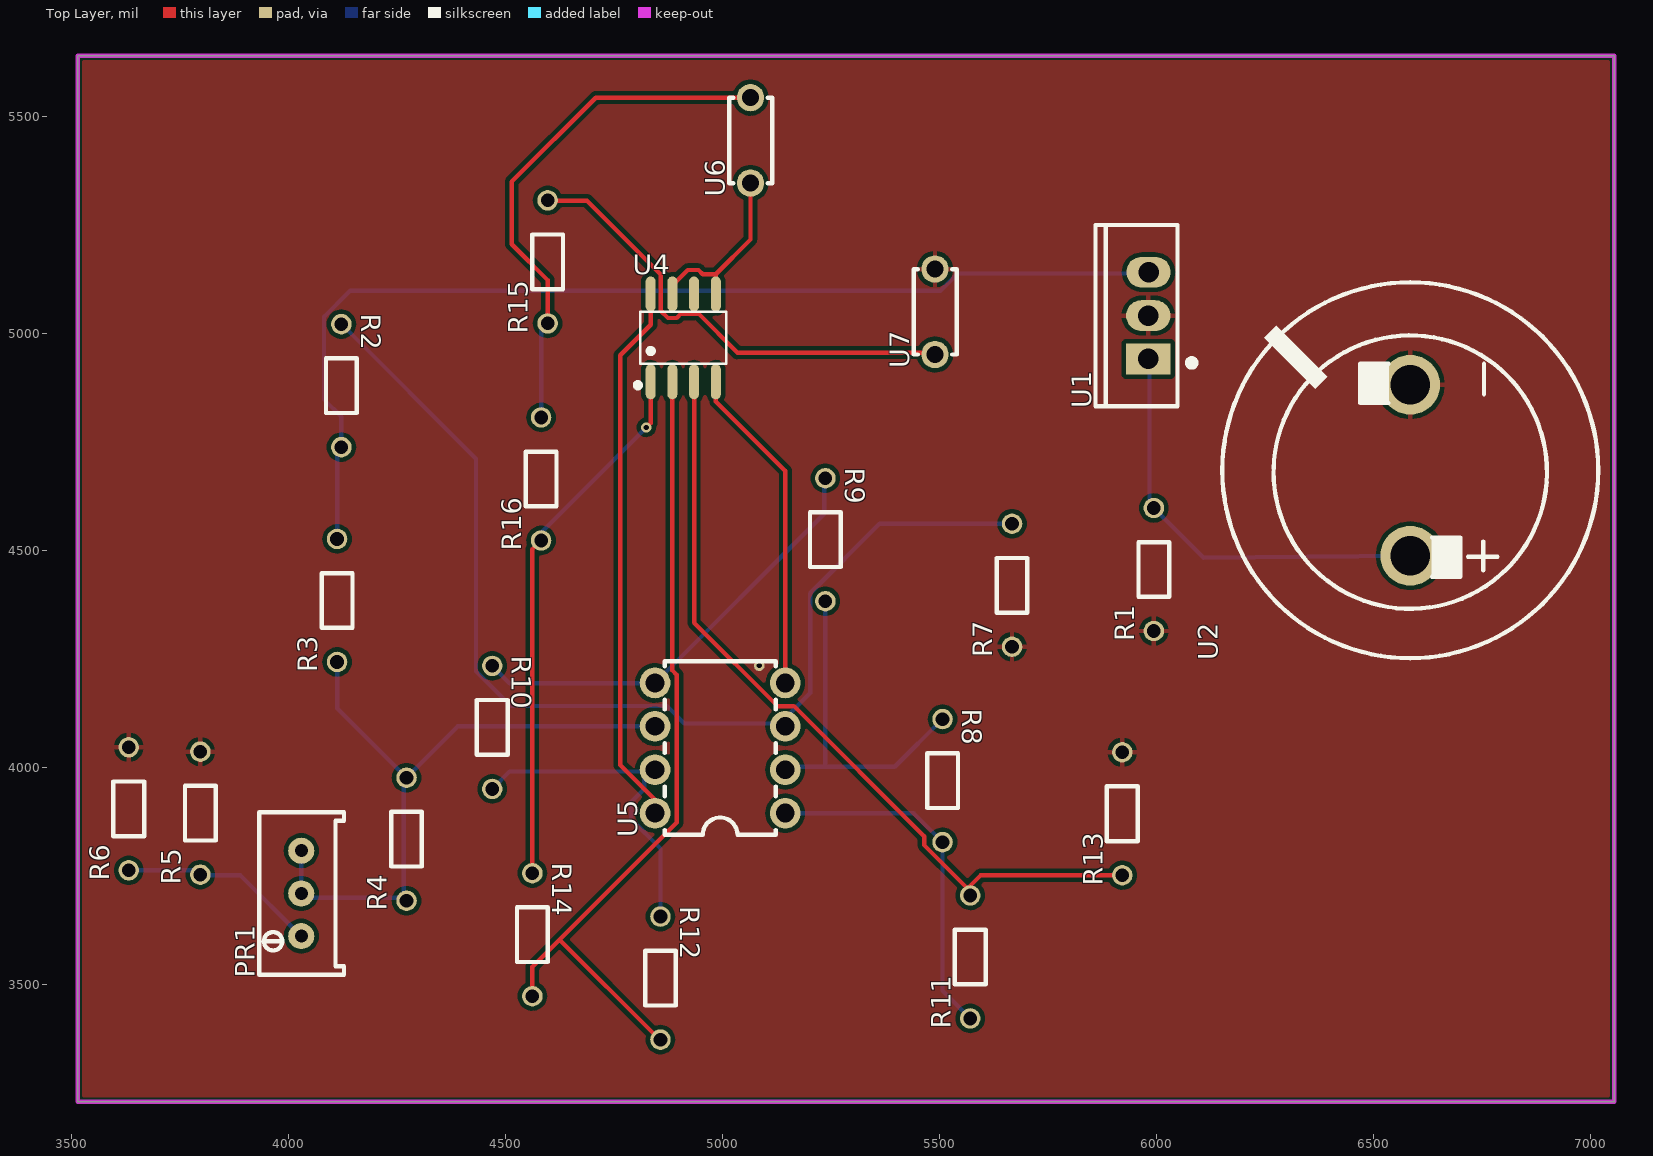
[diagram p0: Top Layer view]
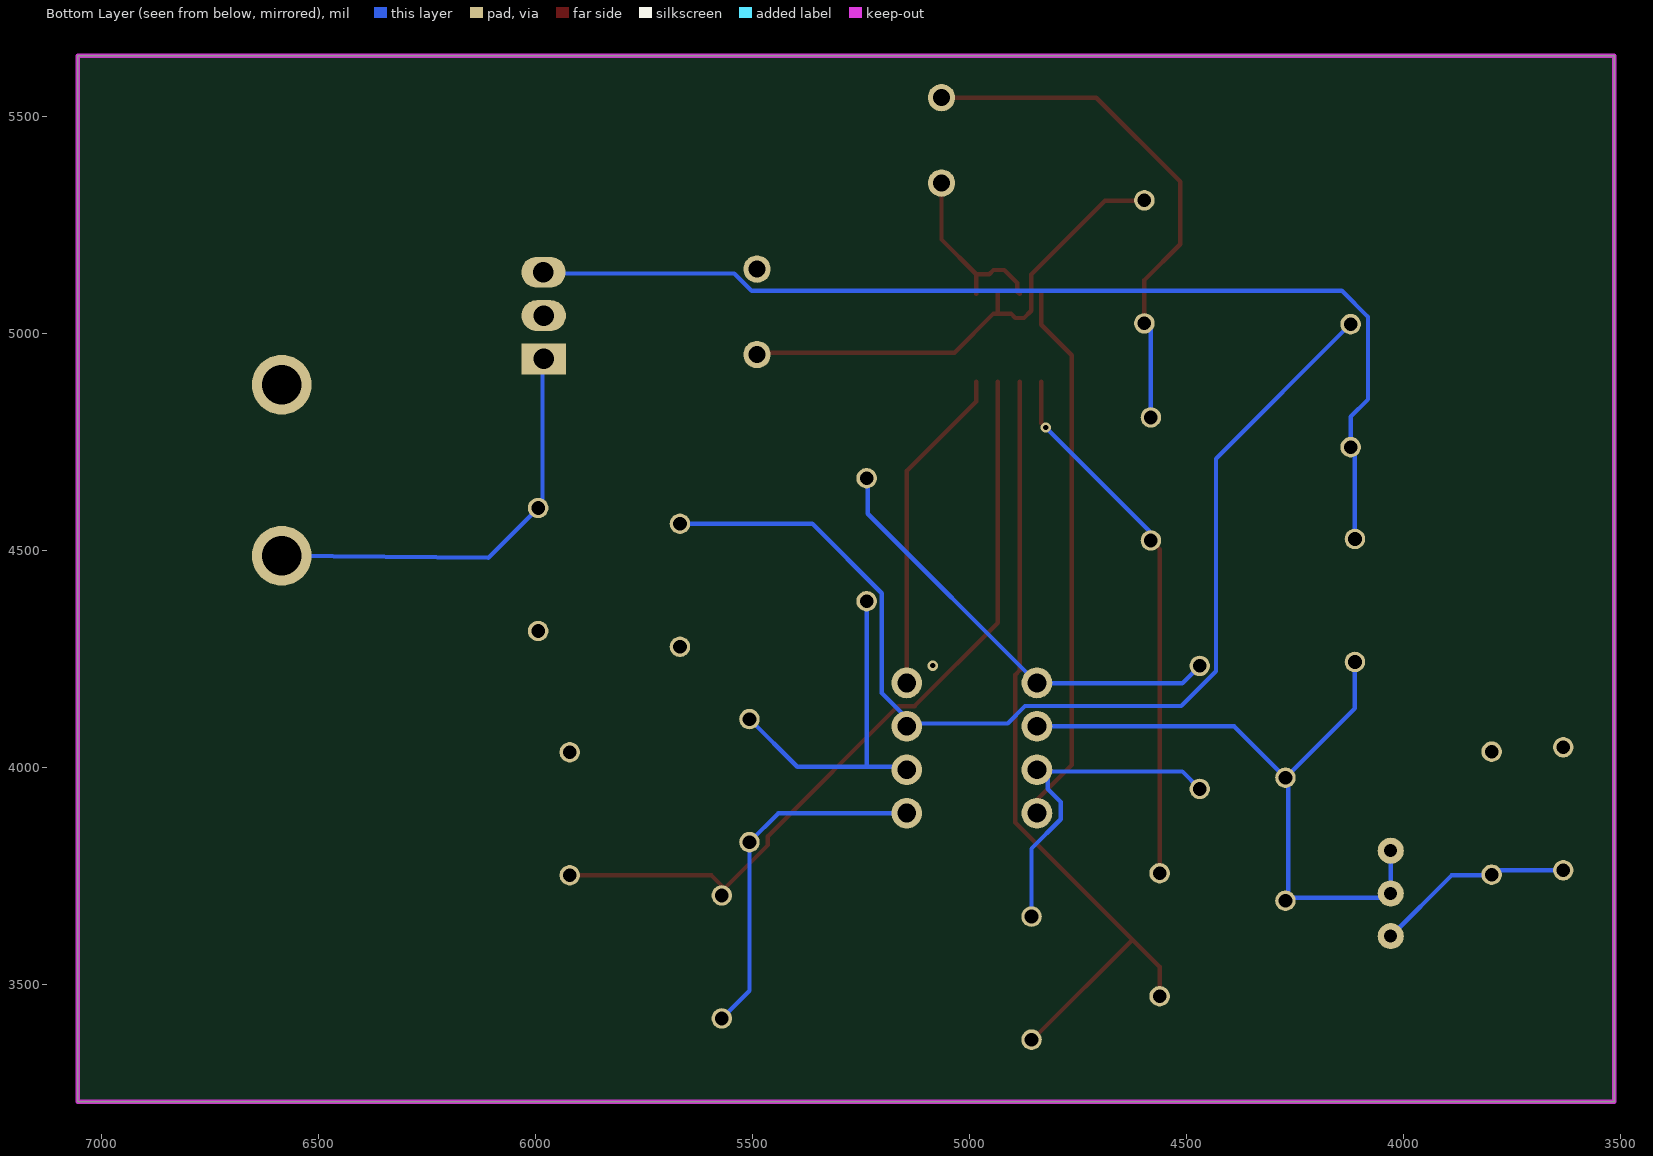
[diagram p1: Bottom Layer view, seen from below]
# Altium PCB MISC51804.pcbdoc
Units mil, origin at the board's own origin, x right, y up, seen from the top; angles counter-clockwise.
Board outline 3540 x 2410 mil, 2 copper layers (Top Layer, Bottom Layer), stack 62.206 mil thick; 23 components, 18 nets, 60 pads, 2 vias.

## Layer stack, top to bottom
Top Solder Mask Layer: solder mask 0.394, Dk 3.3
Top Layer: signal copper 1.379
Dielectric1: surface 59.449, FR4, Dk 4.5
Bottom Layer: signal copper 1.378
Bottom Solder Mask Layer: solder mask 0.394, Dk 3.3

## Board outline
3515,5640 3515,3230 7055,3230 7055,5640

## Design rules (kind name [scope] priority, off if disabled: settings)
BoardOutlineClearance copperThickness2oz_1 [All] p2 off: genericclearance=7.99 ignorepadtopadclearanceinfootprint=FALSE except(0: Arc-SplitContinuation Track-SplitContinuation SMDPad-SplitContinuation THPad-SplitContinuation Via-SplitContinuation Fill-SplitContinuation Region-SplitContinuation Poly-SplitContinuation Text-SplitContinuation Hole-SplitContinuation; 5.98: Arc-CutoutEdge SMDPad-CutoutEdge THPad-CutoutEdge Via-CutoutEdge Fill-CutoutEdge Region-CutoutEdge Text-CutoutEdge; 6.93: Hole-OutlineEdge Hole-CutoutEdge; 10: Poly-OutlineEdge Poly-CutoutEdge; 11.81: Arc-OutlineEdge Track-OutlineEdge SMDPad-OutlineEdge THPad-OutlineEdge Via-OutlineEdge Fill-OutlineEdge Region-OutlineEdge Text-OutlineEdge Track-CutoutEdge)
BoardOutlineClearance copperThickness1oz_1 [All] p4: genericclearance=4.02 ignorepadtopadclearanceinfootprint=FALSE except(0: Arc-SplitContinuation Track-SplitContinuation SMDPad-SplitContinuation THPad-SplitContinuation Via-SplitContinuation Fill-SplitContinuation Region-SplitContinuation Poly-SplitContinuation Text-SplitContinuation Hole-SplitContinuation; 6: SMDPad-CutoutEdge THPad-CutoutEdge Via-CutoutEdge Fill-CutoutEdge Region-CutoutEdge Text-CutoutEdge; 6.93: Hole-OutlineEdge Hole-CutoutEdge; 10: Poly-OutlineEdge Poly-CutoutEdge; 11.8: Arc-OutlineEdge Track-OutlineEdge SMDPad-OutlineEdge THPad-OutlineEdge Via-OutlineEdge Fill-OutlineEdge Region-OutlineEdge Text-OutlineEdge; 11.81: Arc-CutoutEdge Track-CutoutEdge)
Clearance copperThickness2oz [All] p1 off: gap=7.99 ignorepadtopadclearanceinfootprint=FALSE except(5.98: SMDPad-Track SMDPad-SMDPad THPad-Track SMDPad-THPad THPad-THPad Track-Via SMDPad-Via THPad-Via Via-Via Fill-Track Region-Track Fill-SMDPad Region-SMDPad Fill-THPad Region-THPad Fill-Via Region-Via Fill-Fill Fill-Region Region-Region Arc-Track Arc-SMDPad Arc-THPad Arc-Via Fill-Arc Region-Arc Arc-Arc Text-Track SMDPad-Text Text-THPad Text-Via Fill-Text Region-Text Arc-Text Text-Text; 6.93: Hole-Track Hole-SMDPad Hole-THPad Hole-Via Fill-Hole Region-Hole Hole-Arc Hole-Text; 10: Poly-Track Poly-SMDPad Poly-THPad Poly-Via Poly-Fill Poly-Region Poly-Poly Poly-Arc Poly-Text Poly-Hole)
Clearance copperThickness1oz [All] p3: gap=4.02 ignorepadtopadclearanceinfootprint=FALSE except(5.98: SMDPad-Track SMDPad-SMDPad THPad-Track SMDPad-THPad THPad-THPad Track-Via SMDPad-Via THPad-Via Via-Via Fill-Track Region-Track Fill-SMDPad Region-SMDPad Fill-THPad Region-THPad Fill-Via Region-Via Fill-Fill Fill-Region Region-Region; 6: Arc-Track Arc-SMDPad Arc-THPad Arc-Via Fill-Arc Region-Arc Arc-Arc Text-Track SMDPad-Text Text-THPad Text-Via Fill-Text Region-Text Arc-Text Text-Text; 6.93: Hole-Track Hole-SMDPad Hole-THPad Hole-Via Fill-Hole Region-Hole Hole-Arc Hole-Text; 10: Poly-Track Poly-SMDPad Poly-THPad Poly-Via Poly-Fill Poly-Region Poly-Poly Poly-Arc Poly-Text Poly-Hole)
DiffPairsRouting differentialPair [All] p1: maxlimit=6 minlimit=6 mostfreqgap=6 toplayer_minwidth=5 toplayer_prefwidth=10 toplayer_maxwidth=100 toplayer_mingap=6 toplayer_prefgap=6 toplayer_maxgap=6 bottomlayer_minwidth=5 bottomlayer_prefwidth=10 bottomlayer_maxwidth=100 bottomlayer_mingap=6 bottomlayer_prefgap=6 bottomlayer_maxgap=6 maxuncoupledlength=10
HoleToHoleClearance otherClearance [All] p1: gap=11.81 allowstackedmicrovias=TRUE
Length netLength [All] p1: minlimit=0 maxlimit=0
MatchedLengths netLengthTolerance [All] p1: tolerance=1000
PasteMaskExpansion pasteMaskExpansion [All] p1: expansion=0
PlaneConnect innerPlane [All] p1: planeconnectstyle=Relief reliefexpansion=20 reliefentries=4 reliefconductorwidth=10 reliefairgap=10
PolygonConnect copperRegion [(InNet('GND'))] p1: connectstyle=Relief reliefconductorwidth=10 reliefentries=4 polygonreliefangle="90 Angle" airgapwidth=10 via.connectstyle=Relief via.reliefconductorwidth=10 via.reliefentries=4 via.polygonreliefangle="90 Angle" via.airgapwidth=10
RoutingVias viaSize [All] p1: holewidth=12.01 width=24.02 viastyle="Through Hole" minholewidth=11.81 minwidth=19.68 maxholewidth=248.03 maxwidth=393.7
SolderMaskExpansion solderMaskExpansion [IsVia] p1: expansion=-1000 istentingtop=TRUE
SolderMaskExpansion solderMaskExpansion [All] p2: expansion=2 istentingtop=FALSE
Width copperThickness2oz_2 [All] p1 off: maxlimit=100 minlimit=8 preferedwidth=10
Width copperThickness1oz_2 [All] p2: maxlimit=100 minlimit=5 preferedwidth=10

## Components (designator, comment, footprint, x,y, rotation, side; value= is the part's Value field where it differs from the comment)
PR1 "10kΩ" R_3296 4025,3710 r90 top
R1 "1kΩ" Res_1/8W 5996.73,4456.34 r90 top
R2 "1.1kΩ" Res_1/8W 4120,4880 r270 top
R3 "1.1kΩ" Res_1/8W 4115,4385 r90 top
R4 "1Ω" Res_1/8W 4275,3835 r90 top
R5 "1Ω" Res_1/8W 3800,3895 r90 top
R6 "1Ω" Res_1/8W 3635,3905 r90 top
R7 "1.1kΩ" Res_1/8W 5670,4420 r90 top
R8 "500Ω" Res_1/8W 5505,3970 r270 top
R9 "10kΩ" Res_1/8W 5235,4525 r270 top
R10 "400KΩ" Res_1/8W 4467.52,4092.52 r270 top
R11 "100kΩ" Res_1/8W 5573.68,3563.74 r90 top
R12 "100kΩ" Res_1/8W 4855.05,3515 r270 top
R13 "100kΩ" Res_1/8W 5923.97,3893.61 r90 top
R14 "100kΩ" Res_1/8W 4560,3615 r270 top
R15 "1kΩ" Res_1/8W 4600,5165 r90 top
R16 "1kΩ" Res_1/8W 4585,4665 r90 top
U1 "LM7805CT" TO-220-3_L10.0-W4.5-P2.54-L 5981.73,5041.34 r90 top
U2 "820uF" CAP-TH_BD22.0-P10.00-D2.2-FD 6585,4685 r90 top
U4 "LM358ADR-EV" SOIC-8_L4.9-W3.9-P1.27-LS6.0-BL 4910,4990 r0 top
U5 "LM358AN/NOPB" PDIP-8_L10.2-W6.5-P2.54-LS7.6-BL 4995,4045 r90 top
U6 "2.4UF" CAP-TH_L5.0-W2.5-P5.00-D1.0 5065,5445 r90 top
U7 "1.2UF" CAP-TH_L5.0-W2.5-P5.00-D1.0 5490,5050 r90 top

## Footprints (in the part's own frame and the unit in brackets; to place one, negate y for a bottom-side part, rotate by r counter-clockwise, add the part's x,y. Pads: shape width x height; smd on the part's side, far side on the other; paste and mask are expansions set on the pad)
CAP-TH_BD22.0-P10.00-D2.2-FD [mm]
  round 3.5 hole 2.3: 1(-5,0) 2(5,0)
  silkscreen extent -11,-11 11,11
CAP-TH_L5.0-W2.5-P5.00-D1.0 [mm]
  round 1.6 hole 1: 1(-2.5,0) 2(2.5,0)
  silkscreen extent -2.5,-1.27 2.5,1.25
PDIP-8_L10.2-W6.5-P2.54-LS7.6-BL [mm]
  round 1.8 hole 1.1: 1(-3.81,-3.81) 2(-1.27,-3.81) 3(1.27,-3.81) 4(3.81,-3.81) 5(3.81,3.81) 6(1.27,3.81) 7(-1.27,3.81) 8(-3.81,3.81)
  silkscreen extent -5.08,-3.25 5.08,3.25
R_3296 [mil]
  round 60 hole 30 paste+0 mask+2: 1(-98.4,-5) 2(0,-5) 3(98.4,-5)
  silkscreen extent -187,-103 187,92
Res_1/8W [mil]
  round 47.2 hole 31.5 paste+0 mask+2: 1(-141.7,2.48) 2(141.7,2.48)
  silkscreen extent -63,-33 63,38
SOIC-8_L4.9-W3.9-P1.27-LS6.0-BL [mm]
  oval 0.588x2.045 smd: 1(-1.905,-2.57) 2(-0.635,-2.57) 3(0.635,-2.57) 4(1.905,-2.57) 5(1.905,2.57) 6(0.635,2.57) 7(-0.635,2.57) 8(-1.905,2.57)
  silkscreen extent -2.8,-2.92 2.53,1.52
TO-220-3_L10.0-W4.5-P2.54-L [mm]
  rect 1.8x2.6 hole 1.2: 1(-2.54,0.005)
  oval 1.8x2.6 hole 1.2: 2(0,0.005)
  oval 1.8x2.6 hole 1.2 copper offset 0,0: 3(2.54,-0.005)
  silkscreen extent -5.3,-2.73 5.3,3.09

## Via types
v1: diameter 24.02, hole 12, Top Layer to Bottom Layer, 2 vias

## Nets (pads, with @x,y where several pads share a name; then routed paths per layer and width w, separated by ;. In a path a pad name is that pad's centre, name@x,y a point inside that pad or via, vN(x,y) a via of type N, cw(c..) or ccw(c..) an arc to the next point about the centre after c; other vN are vias at no path point)
$1N7: PR1.1 R5.1 R6.1 | length 460.1
  Bottom Layer w10: R6.1 3787.53,3763.3 R5.1 3800,3751.6 3890,3751.6 PR1.1
$1N13: R8.1 R9.2 U5.2 | length 792.4
  Bottom Layer w10: U5.2 5150.78,3995 5157.48,4001.7 5237.48,4001.7 ; R9.2 5237.48,4001.7 ; R8.1 5397.48,4001.7 5237.48,4001.7
$1N14: R9.1 R10.1 U5.5 | length 1025.1
  Bottom Layer w10: R10.1 4510,4194.22 4840,4194.22 U5.5 5235,4585 5235,4655 R9.1
$1N17: R11.2 R13.1 U4.3 | length 1838.1
  Top Layer w10: U4.3 4935,4333.57 5126.92,4141.64 5165,4141.64 5465,3841.64 5465,3821.64 R11.2@5565,3721.64 ; R11.2 5565,3711.64 R11.2@5565,3721.64 ; R13.1 5915,3751.64 5595,3751.64 R11.2@5565,3721.64
$1N18: R8.2 R11.1 U5.1 | length 822.8
  Bottom Layer w10: U5.1 5440.78,3895 R8.2 5507.48,3485.76 R11.1
$1N19: R12.2 R14.2 U4.2 | length 1889.8
  Top Layer w10: R14.2 4562.48,3541.04 4625,3603.57 ; R12.2 4857.52,3381.04 4855,3383.57 4845,3383.57 4625,3603.57 ; U4.2 4885,4223.57 4895,4213.57 4895,3873.57 4625,3603.57
$1N20: R10.2 R12.1 U5.7 | length 767.6
  Bottom Layer w10: R10.2 4510,3990.82 U5.7@4820,3990.82 ; U5.7 4840,3990.82 U5.7@4820,3990.82 ; R12.1 4857.52,3813.3 4790,3880.82 4790,3920.82 4820,3950.82 U5.7@4820,3990.82
$1N32: R15.2 U4.6 U7.1 | length 1141.4
  Top Layer w10: R15.2 4608.3,5305.93 4688.3,5305.93 4858.3,5135.93 4858.3,5052.63 4875,5035.93 4895,5035.93 4905,5045.93 4935,5045.93 ; U4.6 4935,5045.93 ; U7.1 5485,4955.93 5035,4955.93 4945,5045.93 4935,5045.93
$1N33: R15.1 R16.2 U6.2 | length 1213.7
  Top Layer w10: R15.1 4597.52,5123.3 4515,5205.82 4515,5350 4708.27,5543.27 U6.2
  Bottom Layer w10: R16.2 4582.52,5008.3 R15.1
$1N36: U4.5 U4.7 U6.1 | length 427.3
  Top Layer w10: U4.7 4890.26,5096.44 4890.26,5116.44 4920.26,5146.44 4945,5146.44 4955,5136.44 4985,5136.44 ; U4.5 4985,5136.44 ; U6.1 5065,5216.44 4985,5136.44
+15V: U4.8 U5.8 | length 1258.3
  Top Layer w10: U4.8 4835,5020 4765,4950 4765,4005.93 4845,3925.93 U5.8
-15V: U4.4 U5.4 | length 760.1
  Top Layer w10: U4.4 4985,4843.56 5145,4683.56 U5.4
GND: R1.1 R5.2 R6.2 R7.1 R13.2 U1.2 U2.2 U7.2
  other v1: 5085,4235
UO1: R2.2 R3.2 U1.3 | length 2473.6
  Bottom Layer w10: R3.2 4112.52,4728.35 R2.2 4122.48,4808.3 4082.48,4848.3 4082.48,5038.3 4142.48,5098.3 5502.47,5098.3 5542.47,5138.3 5972.47,5138.3 U1.3
UO2: R2.1 R7.2 U5.3 | length 2553.7
  Bottom Layer w10: R2.1 4432.48,4711.7 4432.48,4221.7 4512.48,4141.7 4872.48,4141.7 4912.48,4101.7 U5.3@5132.48,4101.7 ; U5.3 5139.18,4095 U5.3@5132.48,4101.7 ; R7.2 5362.47,4561.7 5202.47,4401.7 5202.47,4171.7 U5.3@5132.48,4101.7
UO3: PR1.2 PR1.3 R3.1 R4.1 R4.2 U5.6 | length 1581.7
  Bottom Layer w10: PR1.3 PR1.2 4040,3700 R4.1@4265.82,3700 ; R3.1 4112.52,4136.7 R4.2 ; R4.1 R4.1@4265.82,3700 ; U5.6 4390.82,4095 R4.2 ; R4.1@4265.82,3700 4265.82,3970 R4.2
UO4: R14.1 R16.1 U4.1 | length 1244.3
  Top Layer w10: R14.1 4562.48,4503.25 R16.1 ; v1(4825,4783.56) 4835,4793.56 U4.1
  Bottom Layer w10: R16.1 4585,4533.56 4585,4543.56 v1(4825,4783.56)
VCC: R1.2 U1.1 U2.1 | length 986.8
  Bottom Layer w10: U1.1 5984.26,4938.04 5984.26,4608.04 R1.2 6109.2,4483.1 U2.1

## Polygon pours and split planes (outlines as drawn)
GND on Top Layer (solid, remove dead copper, pour order 0): 3000,5845 3000,3000 7315,3000 7315,5845

## Keep-outs
Board Outline Layer:
  the board outline again, w10